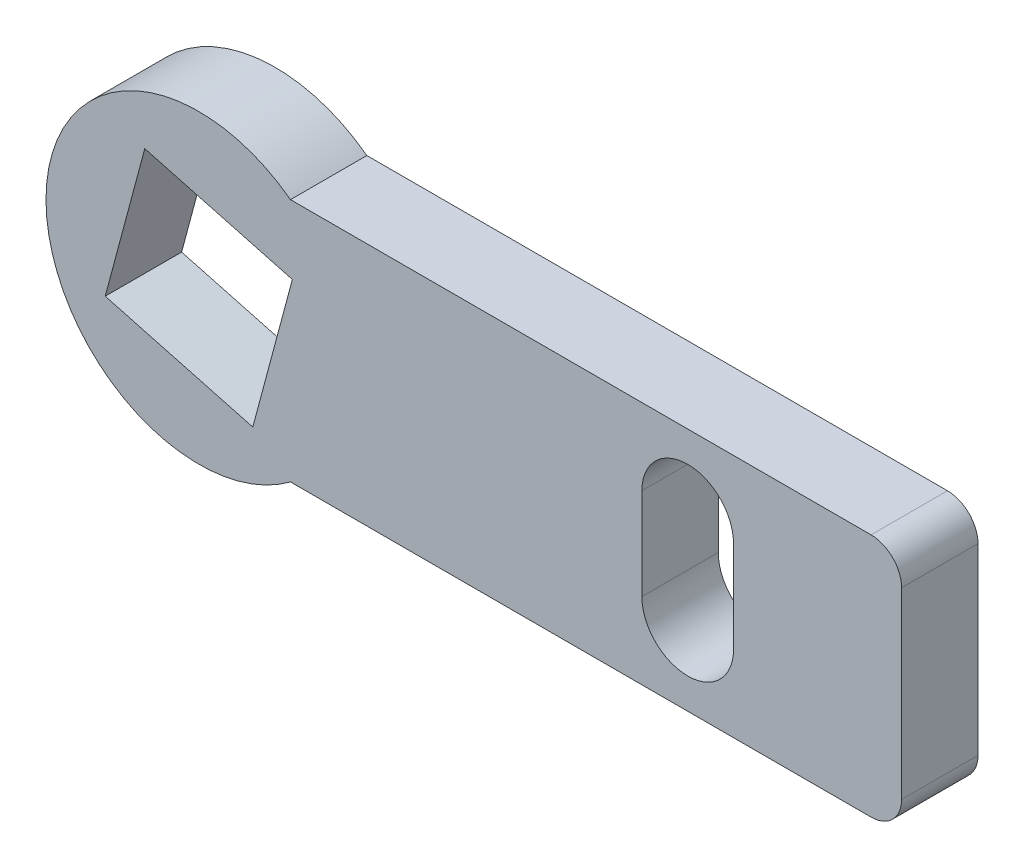
SolidWorks part; units mm, degrees
material "SUS304"
ref_plane "前视基准面" through (0, 0, 0) normal (0, 0, 1) x (1, 0, 0)
ref_plane "上视基准面" through (0, 0, 0) normal (0, 1, 0) x (1, 0, 0)
ref_plane "右视基准面" through (0, 0, 0) normal (1, 0, 0) x (0, 0, -1)
sketch "草图1" plane through (0, 0, 0) normal (0, 0, 1) x (1, 0, 0)
  line L0 (0, 0) -> (27.5009, 0) construction
  line L1 (3, 4) -> (23, 4)
  line L3 (3, -4) -> (23, -4)
  line L4 (23, 4) -> (23, -4)
  arc A0 (3, 4) -> (3, -4) centre (0, 0) ccw
  dimension "D1" = 10
  dimension "D2" = 8
  dimension "D3" = 23
extrude "凸台-拉伸1" add sketch "草图1" along normal mid plane 2.5
sketch "草图2" plane through (0, 0, 1.25) normal (0, 0, 1) x (1, 0, 0)
  line L0 (23, 0) -> (-14.2619, 0) construction
  line L1 (1.7678, -3.0619) -> (3.0619, 1.7678)
  line L2 (1.7678, -3.0619) -> (-3.0619, -1.7678)
  line L3 (-3.0619, -1.7678) -> (-1.7678, 3.0619)
  line L4 (3.0619, 1.7678) -> (-1.7678, 3.0619)
  line L5 (1.7678, -3.0619) -> (-1.7678, 3.0619) construction
  line L6 (-3.0619, -1.7678) -> (3.0619, 1.7678) construction
  line L7 (23, -4) -> (23, 4) construction
  line L8 (16, -1.5) -> (16, 1.5) construction
  line L9 (14.5, -1.5) -> (14.5, 1.5)
  line L10 (17.5, -1.5) -> (17.5, 1.5)
  arc A0 (14.5, -1.5) -> (17.5, -1.5) centre (16, -1.5) ccw
  arc A1 (17.5, 1.5) -> (14.5, 1.5) centre (16, 1.5) ccw
  point P0 (0, 0)
  point P12 (16, 0)
  dimension "D4" = 1.5
  dimension "D1" = 5
  dimension "D2" = 5
  dimension "D3" = 105
  dimension "D5" = 16
  dimension "D6" = 3
extrude "切除-拉伸1" cut sketch "草图2" against normal through all
fillet "圆角1" radius 1 2 edges at (23, -4, 0) (23, 4, 0)
